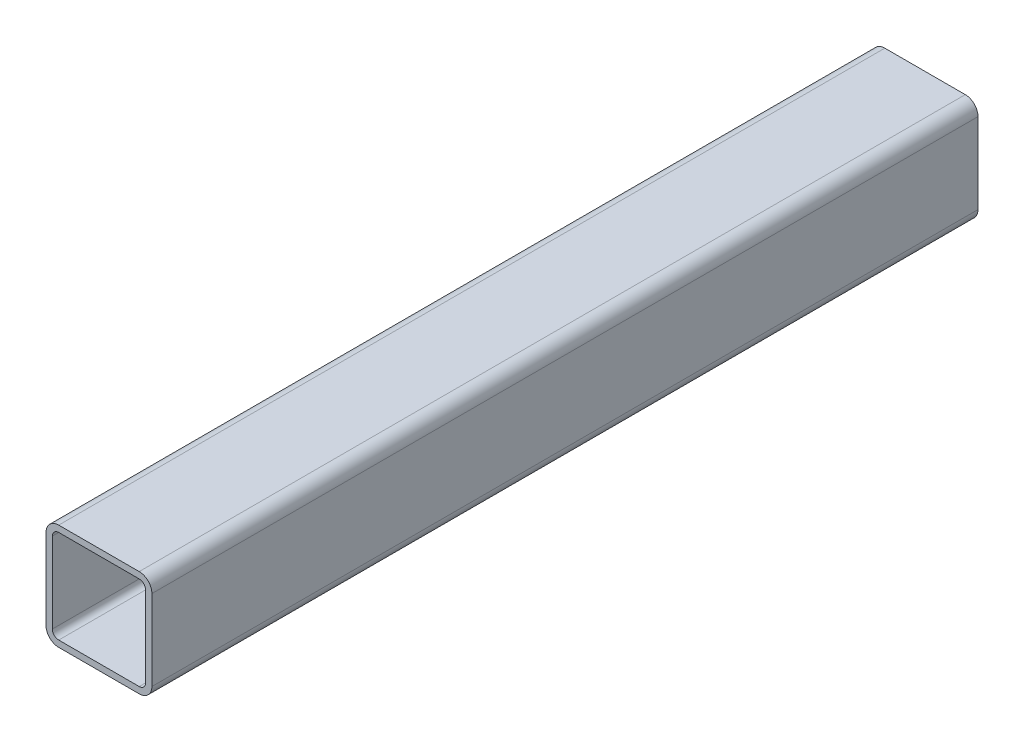
from build123d import *

# Parameters (mm, degrees)
GB_6728_1986_050_X_50_X_3_1_DEPTH = 390


with BuildPart() as part:
    # Sketch1 → Gb／6728-1986方形空心型钢 050 X 50 X 3(1) (new body)
    with BuildSketch(Plane.YX.offset(-195)):
        with BuildLine():
            Line((-19, -25), (19, -25))
            ThreePointArc((19, -25), (23.242640687, -23.242640687), (25, -19))
            Line((25, -19), (25, 19))
            ThreePointArc((25, 19), (23.242640687, 23.242640687), (19, 25))
            Line((19, 25), (-19, 25))
            ThreePointArc((-19, 25), (-23.242640687, 23.242640687), (-25, 19))
            Line((-25, 19), (-25, -19))
            ThreePointArc((-25, -19), (-23.242640687, -23.242640687), (-19, -25))
        make_face()
        with BuildLine():
            Line((-19, -22), (19, -22))
            ThreePointArc((19, -22), (21.121320344, -21.121320344), (22, -19))
            Line((22, -19), (22, 19))
            ThreePointArc((22, 19), (21.121320344, 21.121320344), (19, 22))
            Line((19, 22), (-19, 22))
            ThreePointArc((-19, 22), (-21.121320344, 21.121320344), (-22, 19))
            Line((-22, 19), (-22, -19))
            ThreePointArc((-22, -19), (-21.121320344, -21.121320344), (-19, -22))
        make_face(mode=Mode.SUBTRACT)
    extrude(amount=GB_6728_1986_050_X_50_X_3_1_DEPTH)


solid = part.part
